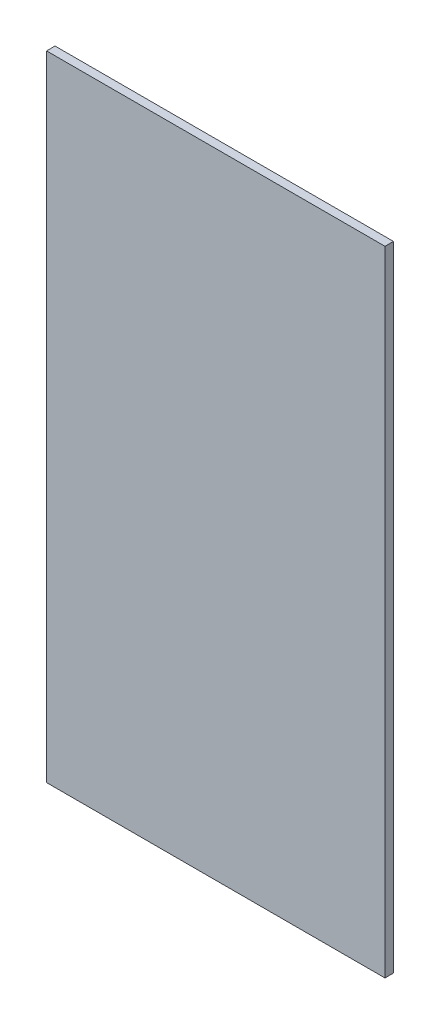
from build123d import *

# Parameters (mm, degrees)
SKETCH1_W           = 400
SKETCH1_H           = 749
BOSS_EXTRUDE1_DEPTH = 5


with BuildPart() as part:
    # Sketch1 → Boss-Extrude1 (new, symmetric)
    with BuildSketch(Plane.XY):
        Rectangle(SKETCH1_W, SKETCH1_H)
    extrude(amount=BOSS_EXTRUDE1_DEPTH, both=True)


solid = part.part
